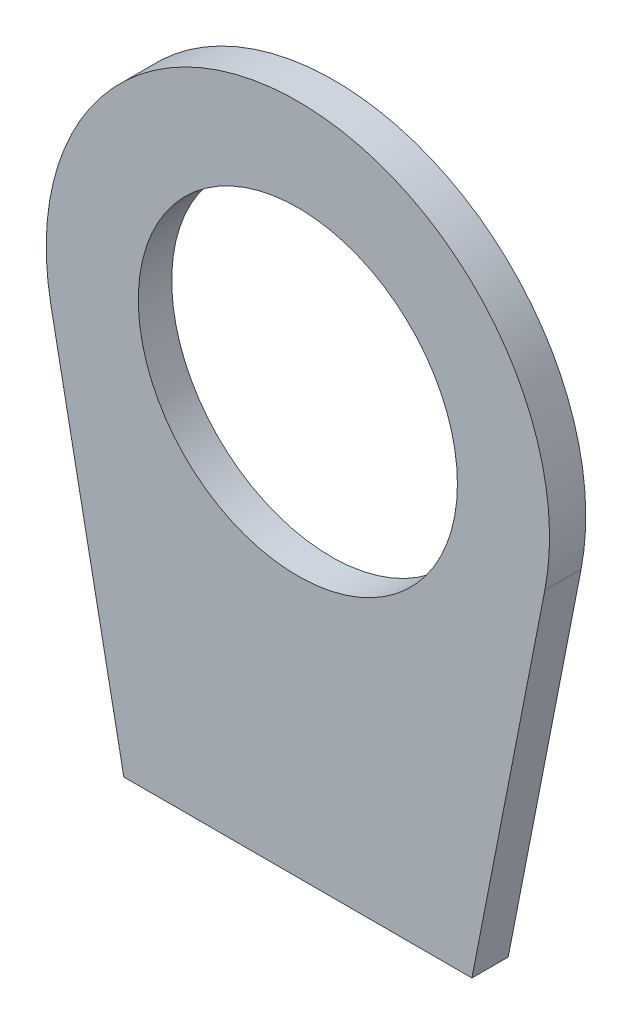
SolidWorks part; units mm, degrees
ref_plane "Front Plane" through (0, 0, 0) normal (0, 0, 1) x (1, 0, 0)
ref_plane "Top Plane" through (0, 0, 0) normal (0, 1, 0) x (1, 0, 0)
ref_plane "Right Plane" through (0, 0, 0) normal (1, 0, 0) x (0, 0, -1)
sketch "Sketch1" plane through (0, 0, 0) normal (0, 0, 1) x (1, 0, 0)
  line L0 (0, -94.8031) -> (0, 121.5186) construction
  line L1 (-120, 0) -> (120, 0)
  line L2 (120, 0) -> (170.2653, 256.6538)
  line L3 (-120, 0) -> (-170.2653, 256.6538)
  arc A0 (170.2653, 256.6538) -> (-170.2653, 256.6538) centre (0, 290) ccw
  circle A1 centre (0, 290) radius 110
  dimension "D1" = 347
  dimension "D5" = 220
  dimension "D2" = 290
  dimension "D3" = 240
  dimension "D4" = 240
extrude "Boss-Extrude1" add sketch "Sketch1" along normal blind 25
sketch "Sketch2" plane through (0, 0, 0) normal (0, 0, 1) x (1, 0, 0)
  circle A0 centre (0, 290) radius 110 construction
  circle A1 centre (0, 290) radius 110
  circle A2 centre (0, 290) radius 123
  dimension "D1" = 246
extrude "Cut-Extrude2" cut sketch "Sketch2" along normal blind 2
